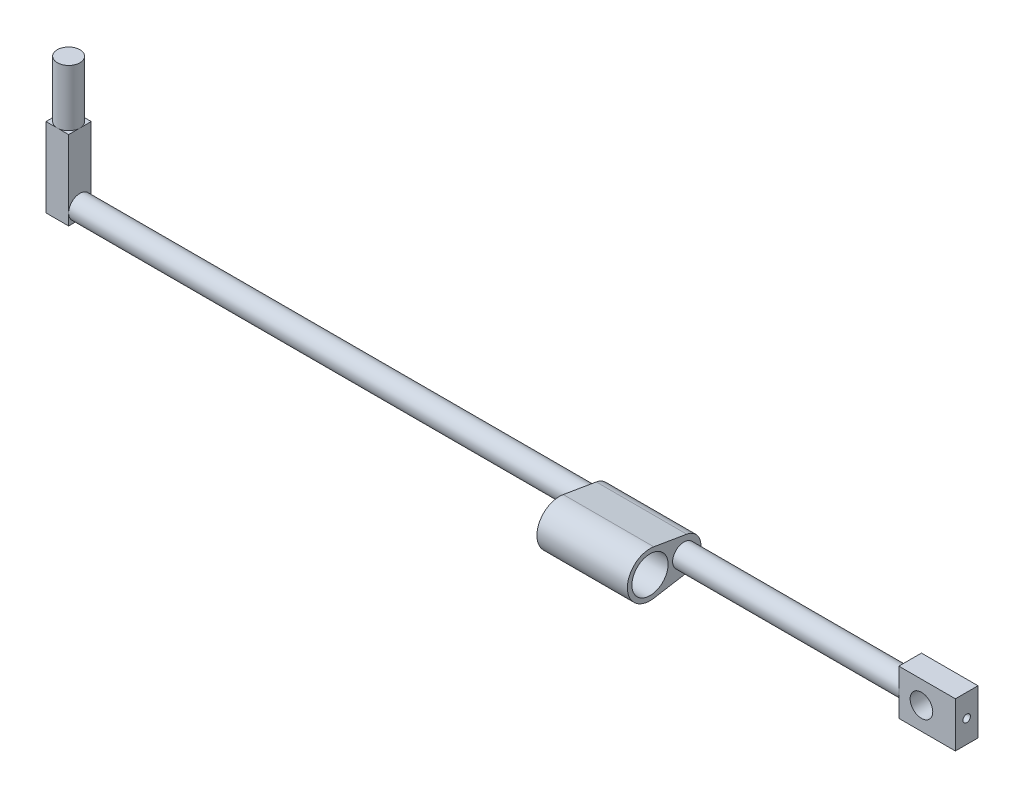
SolidWorks part; units mm, degrees
ref_plane "前视基准面" through (0, 0, 0) normal (0, 0, 1) x (1, 0, 0)
ref_plane "上视基准面" through (0, 0, 0) normal (0, 1, 0) x (1, 0, 0)
ref_plane "右视基准面" through (0, 0, 0) normal (1, 0, 0) x (0, 0, -1)
sketch "草图6" plane through (0, 0, 0) normal (0, 0, 1) x (1, 0, 0)
  line L1 (0, 0) -> (25, 0)
  line L2 (0, 0) -> (0, 20)
  line L3 (0, 20) -> (25, 20)
  line L4 (25, 0) -> (25, 20)
  circle A0 centre (10, 10) radius 5
  dimension "D1" = 10
extrude "凸台-拉伸4" add sketch "草图6" along normal blind 10
sketch "草图7" plane through (0, 0, 0) normal (-1, 0, 0) x (0, 0, 1)
  circle A0 centre (5, 10) radius 5
extrude "凸台-拉伸5" add sketch "草图7" along normal blind 367
hole_wizard "M4 螺纹孔1" positions "草图9" profile "草图8" tap size "M4" standard "Iso"
sketch "草图9" plane through (25, 0, 0) normal (1, 0, 0) x (0, 0, -1)
  point P0 (-5, 10)
sketch "草图8" plane through (25, 10, 5) normal (0, 1, 0) x (0, 0, -1)
  line L0 (0, 0) -> (0, 5.9914)
  line L1 (0, 5.9914) -> (1.65, 5)
  line L2 (1.65, 5) -> (1.65, 0)
  line L5 (1.65, 0) -> (0, 0)
  line L10 (0, 5.9914) -> (-1.65, 5) construction
  line L11 (0, -6.35) -> (0, 107.95) construction
  dimension "螺纹孔钻头直径" = 3.3
  dimension "螺纹孔钻头深度" = 5
  dimension "导头角度" = 118
cosmetic thread "孔螺蚊线2" parameters "D1"=5, "D2"=4
sketch "草图10" plane through (-367, 0, 0) normal (-1, 0, 0) x (0, 0, 1)
  line L0 (10, 10) -> (10, 0) construction
  line L1 (0, 40) -> (10, 40)
  line L2 (0, 15) -> (0, 5)
  line L3 (0, 5) -> (10, 5)
  line L4 (10, 40) -> (10, 5)
  line L7 (0, 15) -> (0, 40)
extrude "凸台-拉伸6" add sketch "草图10" along normal blind 10
sketch "草图11" plane through (0, 40, 0) normal (0, 1, 0) x (1, 0, 0)
  circle A0 centre (-372, -5) radius 5
extrude "凸台-拉伸7" add sketch "草图11" along normal blind 25
ref_plane "基准面1" through (-100, 0, 0) normal (-1, 0, 0) x (0, 0, 1)
sketch "草图12" plane through (-100, 0, 0) normal (-1, 0, 0) x (0, 0, 1)
  line L0 (3.75, 17.3951) -> (18.3333, 19.8601)
  line L1 (3.75, 2.6049) -> (18.3333, 0.1399)
  circle A0 centre (20, 10) radius 8
  arc A3 (3.75, 17.3951) -> (3.75, 2.6049) centre (5, 10) ccw
  arc A4 (18.3333, 0.1399) -> (18.3333, 19.8601) centre (20, 10) ccw
extrude "凸台-拉伸8" add sketch "草图12" along normal blind 40
